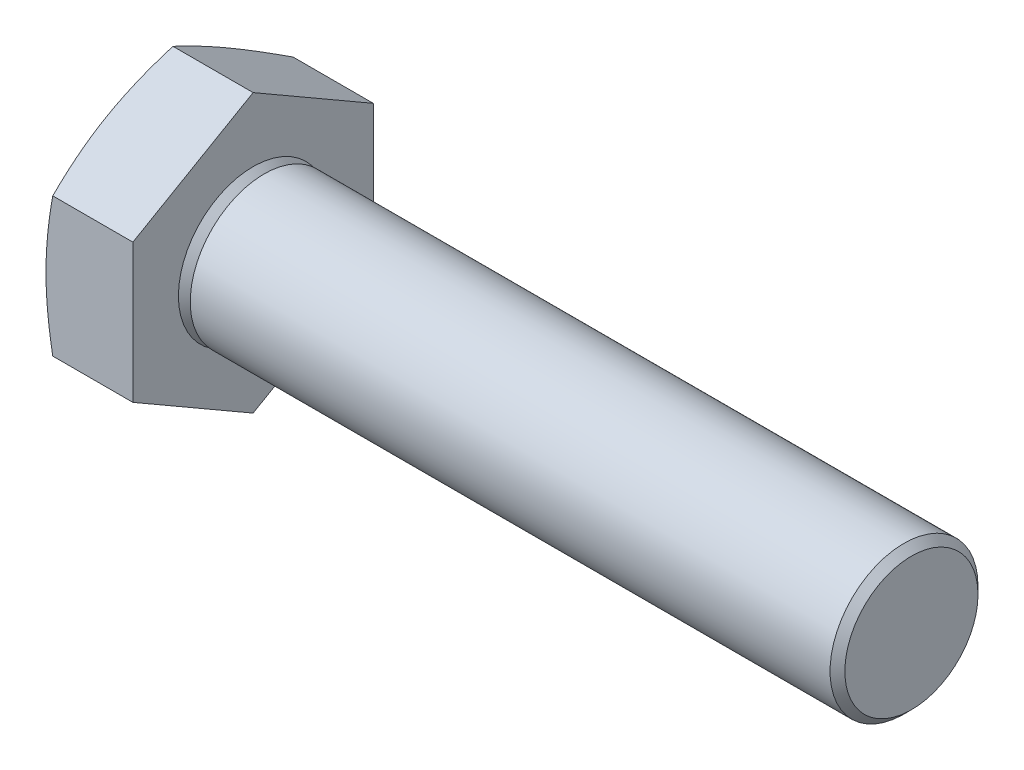
SolidWorks part; units mm, degrees
ref_plane "Front" through (0, 0, 0) normal (0, 0, 1) x (1, 0, 0)
ref_plane "Top" through (0, 0, 0) normal (0, 1, 0) x (1, 0, 0)
ref_plane "Right" through (0, 0, 0) normal (1, 0, 0) x (0, 0, -1)
other "Configuration Table"
sketch "Sketch2" plane through (0, 0, 0) normal (1, 0, 0) x (0, 0, -1)
  line L1 (6.5, -3.7528) -> (6.5, 3.7528)
  line L2 (6.5, 3.7528) -> (0, 7.5056)
  line L3 (0, 7.5056) -> (-6.5, 3.7528)
  line L4 (-6.5, 3.7528) -> (-6.5, -3.7528)
  line L5 (-6.5, -3.7528) -> (0, -7.5056)
  line L6 (0, -7.5056) -> (6.5, -3.7528)
  circle A0 centre (0, 0) radius 6.5 construction
extrude "BaseHead" add sketch "Sketch2" along normal blind 5.3
sketch "Sketch3" plane through (0, 0, 0) normal (0, 0, 1) x (1, 0, 0)
  line L0 (5.3, 7.5056) -> (5.3, 3.44)
  line L2 (5.3, 3.44) -> (4.7, 4.04)
  line L3 (4.7, 4.04) -> (4.7, 7.5056)
  line L5 (4.7, 7.5056) -> (5.3, 7.5056)
  line L6 (-0.9571, 0) -> (7.6478, 0) construction
  line L7 (5.3, 7.5056) -> (0, 7.5056) construction
  dimension "D1" = 45
  dimension "c" = 0.6
  dimension "Dw" = 6.88
revolve "BearingFace" cut sketch "Sketch3" angle 360 about L6
sketch "Sketch4" plane through (0, 0, 0) normal (0, 0, 1) x (1, 0, 0)
  line L0 (-0.4935, 0) -> (3.5626, 0) construction
  line L2 (0, 7.5056) -> (0.366, 7.5056)
  line L4 (0.366, 7.5056) -> (0, 6.5)
  line L6 (0, 6.5) -> (0, 7.5056)
  line L7 (4.7, 7.5056) -> (0, 7.5056) construction
revolve "HeadChamfer" cut sketch "Sketch4" angle 360 about L0
sketch "Sketch5" plane through (5.3, 0, 0) normal (1, 0, 0) x (0, 0, -1)
  circle A0 centre (0, 0) radius 4
extrude "BaseBody" add sketch "Sketch5" along normal blind 35
cosmetic thread "ThreadCosmetic1" parameters "D2"=7
chamfer "Chamfer1" distance 0.4 angle 45 1 edges at (40.3, 0, -4)
fillet "HeadFillet" [suppressed] radius 0.4
sketch "Sketch6" plane through (0, 0, 0) normal (0, 0, 1) x (1, 0, 0)
  line L0 (3.65, 3) -> (4.15, 3)
  line L1 (4.15, 3) -> (4.15, 2.5)
  line L2 (4.15, 2.5) -> (3.9, 2.067)
  line L3 (3.9, 2.067) -> (3.65, 2.5)
  line L4 (3.65, 2.5) -> (3.65, 3)
  line L5 (43.4, 2.5) -> (3.65, 2.5) construction
  line L6 (3.65, -3.44) -> (3.65, 3.44) construction
revolve "Cut-Revolve10" [suppressed] cut sketch "Sketch6" angle 360 about axis through (-0.9571, 0, 0) along (1, 0, 0)
pattern_linear "LPattern10" [suppressed] count 58
equation "\"D2@Sketch4\" = \"s@Sketch2\""
equation "\"D1@Chamfer1\" = 0.05 * \"d@Sketch5\""
equation "\"D1@Sketch6\" =  ( \"d@Sketch5\" - \"D2@ThreadCosmetic1\" )  / 2"
equation "\"pitch@LPattern10\" = \"D1@Sketch6\" * 1.2"
equation "\"D1@LPattern10\" = \"l@BaseBody\" / \"pitch@LPattern10\""
